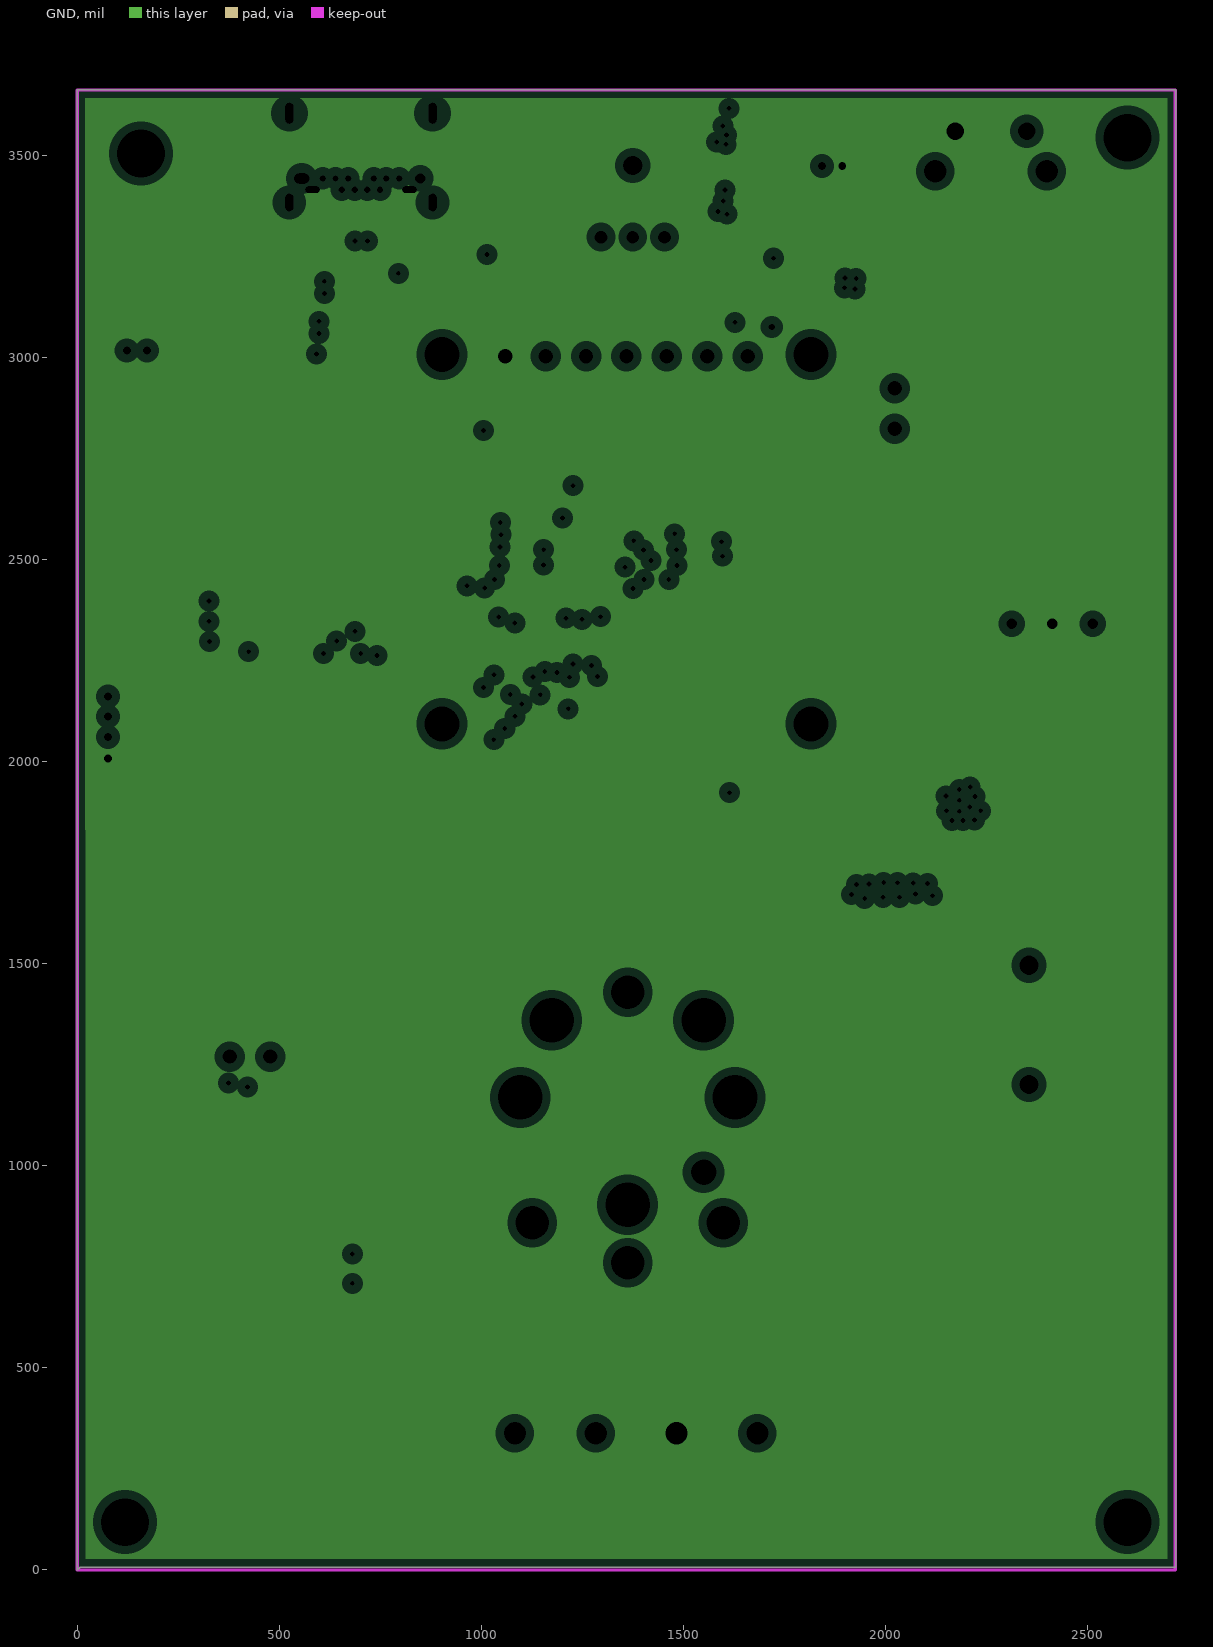
[diagram p0: GND, clearances drawn from the general rule]
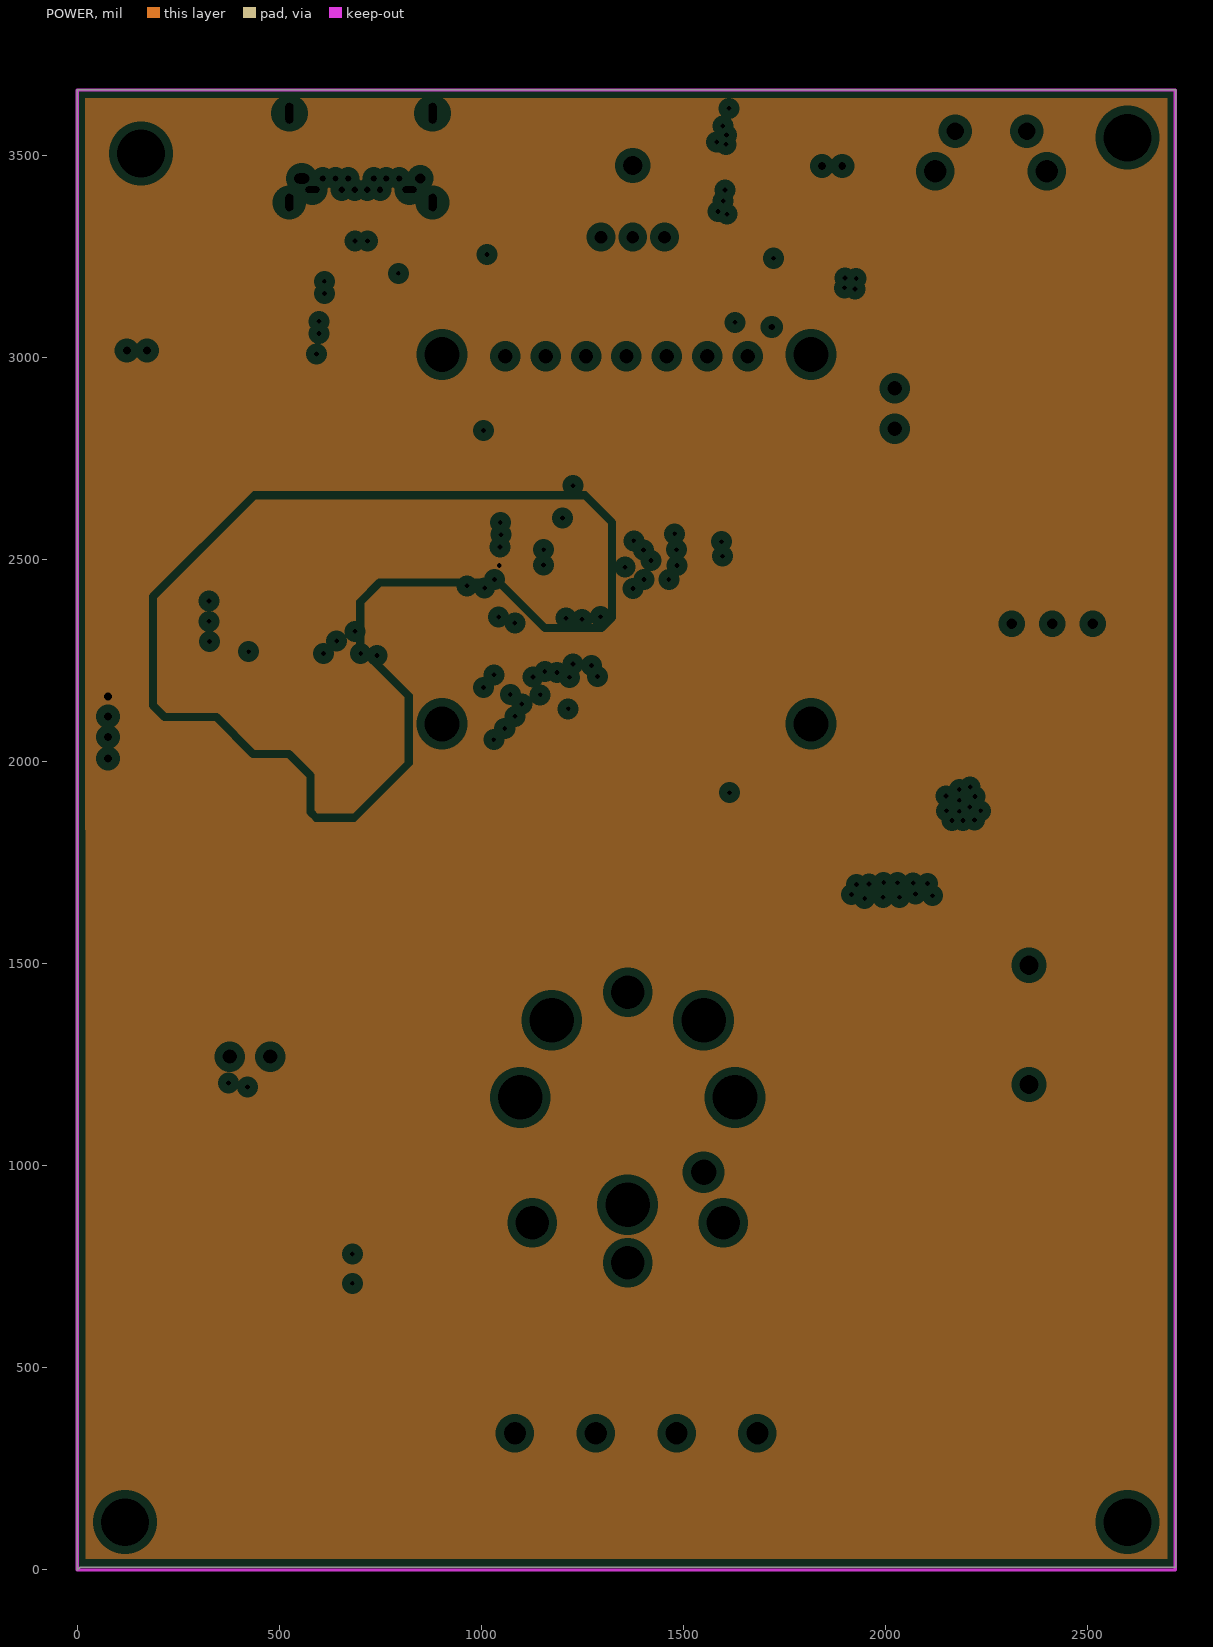
[diagram p1: POWER, clearances drawn from the general rule]
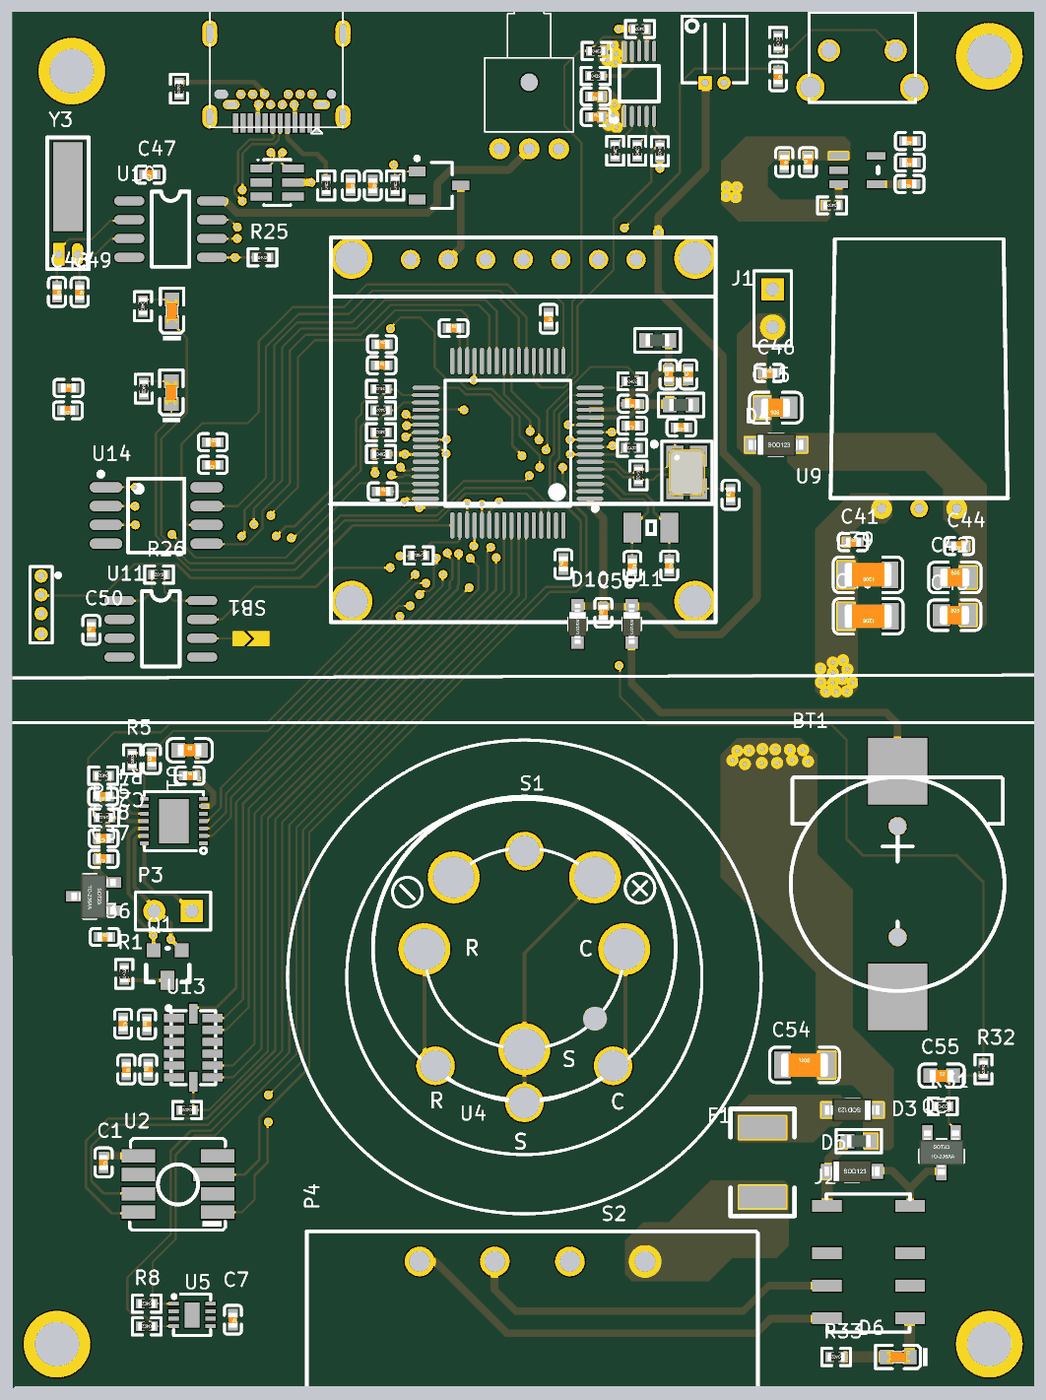
[diagram p2: 3D render of the assembled board from above, using the file's embedded part models]
# Altium PCB MISC105202.PcbDoc (part 2 of 3)
## Footprints (in the part's own frame and the unit in brackets; to place one, negate y for a bottom-side part, rotate by r counter-clockwise, add the part's x,y. Pads: shape width x height; smd on the part's side, far side on the other; paste and mask are expansions set on the pad) (continued)
SOT23-5 [mil]
  rect 20x50 smd: 1(74.8,100) 2(37.4,100) 3(0,100) 4(0,0) 5(74.8,0)
  silkscreen extent 30,-5 45,-5
SOT23-6 [mm] "SOT-23/SC-74A; 5 Leads; Body 3.1 x 3 mm, inc. leads (LxW max)"
  rect 0.55x1.45 smd: 1(-0.95,-1.075) 2(0,-1.075) 3(0.95,-1.075) 4(0.95,1.075) 5(0,1.075) 6(-0.95,1.075)
  silkscreen extent -1.57,-1.35 1.55,0.9
SOT-23 [mil]
  rect 36x36 smd: 1(0,0) 2(75,0)
  rect 36x50 smd: 3(38,80)
  silkscreen extent -20,-5 95,85
SOT-23(SOT-23-3) [mm]
  rect 1.25x0.7 smd: 1(1.25,-0.95) 2(1.25,0.95) 3(-1.25,0)
  silkscreen extent -0.65,-1.46 0.9,1.46, body extent -1.5,-1.5 1.5,1.5, height 1.3
SOT-23-3L [mm] "http://www.aosmd.com/res/packaging_information/SOT-23-3L.pdf"
  rect 1.15x0.65 smd: 1(1.475,-0.95) 2(1.475,0.95) 3(-1.475,0)
  silkscreen extent -0.9,-1.95 1.6,1.55, body extent -0.9,-1.55 0.9,1.55, height 1.25
USB_TYPEC [mm]
  oval 1x1.8 hole 0.5 slot 1.3 at 90 deg: 0(-4.5,-2.805) 0(4.5,-2.805)
  oval 1x1.6 hole 0.5 slot 1.1 at 90 deg: 0(-4.5,2.805) 0(4.5,2.805)
  round 0.61 hole 0.65 unplated: 0(-3.725,1.295)
  oval 0.64x0 hole 0.64 slot 0.95 at 0 deg unplated: 0(3.725,1.295)
  rect 0.35x1.3 smd: A1(-2.75,3.243) A2(-2.25,3.243) A3(-1.75,3.243) A4(-1.25,3.243) A5(-0.75,3.243) A6(-0.25,3.243) A7(0.25,3.243) A8(0.75,3.243) A9(1.25,3.243) A10(1.75,3.243) A11(2.25,3.243) A12(2.75,3.243)
  oval 1.14x0.64 hole 0.4 slot 0.9 at 0 deg: B1(3.05,1.995)
  round 0.65 hole 0.4: B2(2.4,1.295) B3(1.6,1.295) B4(1.2,1.995) B8(-0.8,1.295) B10(-1.6,1.295) B11(-2.4,1.295)
  round 0.64 hole 0.4: B5(0.8,1.295) B6(0.4,1.995) B7(-0.4,1.995) B9(-1.2,1.995)
  oval 1.15x0.65 hole 0.4 slot 0.9 at 0 deg: B12(-3.05,1.995)
  silkscreen extent -4.5,-6.46 4.5,3.96
WSON-14 [mm]
  rect 2x3 smd: 0(0,0)
  rect 0.6x0.254 smd: 1(-2,1.5) 2(-2,1) 3(-2,0.5) 4(-2,0) 5(-2,-0.5) 6(-2,-1) 7(-2,-1.5) 8(2,-1.5) 9(2,-1) 10(2,-0.5) 11(2,0) 12(2,0.5) 13(2,1) 14(2,1.5)
  silkscreen extent -2.2,-2 2,2.2
ZY78xxLS-1000 [mm]
  round 1.2 hole 0.65: 1(-2.54,0) 2(0,0) 3(2.54,0)
  silkscreen extent -6,0.69 6,18.2

## Part data
BT1: library part Battery, "Multicell Battery"
C1 C3 C4 C5 C7 C8 C10 C11 C12 C13 C14 C15 C16 C17 C18 C21 C22 C23 C24 C25 C26 C28 C31 C35 C47 C48 C49 C50 C51 C53: library part "Cap Semi", "Capacitor (Semiconductor SIM Model)"
C2: library part "0603 1uF (105) 10% 50V", "贴片电容"
C6 C9 C20 C27 C30 C52: library part "Cap Pol1", "Polarized Capacitor (Radial)"
C19: library part "0402 10nF (103) 10% 50V", "贴片电容"
C29 C33 C37 C41 C44 C46: library part "0402 100nF (104) 10% 16V", "贴片电容"
C32 C34 C36 C38: library part "0402 10uF (106) 20% 6.3V", "贴片电容"
C39 C40 C54: library part "1206 10uF (106) 10% 50V", "贴片电容"
C42 C43 C45: library part "0805 22uF (226) 20% 25V", "贴片电容"
C55: library part "0603 22uF (226) 20% 6.3V", "贴片电容"
C56: library part CAP, "Capacitor"
D1 D6: library part "0603 绿灯", "发光二极管"
D2: library part "0603 红灯", "发光二极管"
D3 D4 D5: library part "SOD-123 B5819W  SL", "肖特基二极管"
D10 D11: library part "SOD-323 1N4148WS T4", "二极管"
F1: library part "Fuse 2", "Fuse"
J1 P1 P3: library part "Header 2", "Header, 2-Pin"
L1 L2 L3: library part "0603 10uH 10%", "贴片电感"
OLED1: library part OLED_0.96
P2 P4: library part "Header 4", "Header, 4-Pin"
Q1: library part JFET
Q2: library part "AO3401A P道沟 X13A15 SOT-23", "MOS(场效应管)"
Q3: library part "SOT-23 SS8050 Y1", "三极管"
R1 R4: library part "0603 1.1KΩ (1101) 1%", "贴片电阻"
R2 R3 R5 R6 R8 R9 R10 R11 R12 R13 R14 R16 R17 R18 R19 R20 R21 R22 R23 R24 R25 R26 R27 R28 R29 R33: library part Reszte, "Resistor"
R7 R30: library part "0402 120Ω (1200) 1%", "贴片电阻"
R15: library part "0603 100Ω (1000) 1%", "贴片电阻"
R31: library part "0402 5.1KΩ (5101) 1%", "贴片电阻"
R32: library part "0402 680Ω (6800) 1%", "贴片电阻"
S2: library part 4NT
S3: library part SW-PB
SB1: library part JP2
U1: library part LMP91002
U3: library part TPS76901HDB
U6: "ARM"
U7: library part TPD4E001
U8: library part REF31xx
U9: library part ZY78xxLS
U11: library part SP706
U14: library part W25Q128FV
USB1: library part USB_Type_C_Receptacle
Y1: library part CRYSTAL_32K, "Crystal"
Y2: library part "SMD-3225_4P  16MHZ 9PF 10PPM", "贴片晶振"
Y3: library part XTAL_2P, "Crystal Oscillator"

## Free pads (board coordinates)
  round 177.17 hole 118.11: 0(118.11,118.11) 0(157.48,3503.94) 0(2598.43,118.11) 0(2598.43,3543.31)

## Via types
v1: diameter 24, hole 12, Top Layer to Bottom Layer, 107 vias
v2: diameter 30, hole 15, Top Layer to Bottom Layer, 1 vias

## Nets (pads, with @x,y where several pads share a name; then routed paths per layer and width w, separated by ;. In a path a pad name is that pad's centre, name@x,y a point inside that pad or via, vN(x,y) a via of type N, cw(c..) or ccw(c..) an arc to the next point about the centre after c; other vN are vias at no path point)
3V3: C1.1 C3.2 C4.2 C7.2 C9.1 C10.2 C11.2 C12.2 C13.2 C14.2 C17.2 C18.2 C20.1 C21.2 C27.1 C28.2 C30.1 C31.2 C33.2 C34.2 C47.2 C50.2 D10.1 L1.2 M1.2 M1.11 P2.1 Q2.2 R8.2 R9.2 R10.1 R11.2 R12.2 R16.2 R17.2 R19.1 R20.2 R21.2 R24.2 R25.2 R33.2 U1.6 U2.5 U3.5 U5.5 U6.19 U6.32 U6.64 U10.1 U11.2 U13.1 U13.6 U14.8 | length 272
  Top Layer w6: C1.1@245.67,617.72 C1.1@246.46,618.5
  Top Layer w12: C4.2@491,1628 C3.2@491,1687
  Top Layer w15: C4.2@487.73,1630 534,1583.73 534,1558 525,1549 U1.6@505,1549
  Top Layer w20: C1.1@246.46,618.5 U2.5@334.46,618.5
+5: C45.2 C46.1 C51.2 C52.1 D4.2 J1.2 U12.1 | length 898.7
  Top Layer w15: C51.2@1567.73,3382 C52.1@1567.73,3434.27 ; C51.2@1578.88,3384.12 U12.1@1625,3384.12
  Bottom Layer w20: v1@1599,3379 v1@1599,3384
  Bottom Layer w40: v1@1597,3379 1597,3279 1755,3121 1863,3121 1923,3061 1923,2922 J1.2@2022,2823
  other v1: 1607,3354 1585,3361 1598,3387 1602,3414
ADC1_IN1: C5.2 R5.2 U6.8 | length 1810.6
  Top Layer w6: R5.2@318.5,1690.35 C5.2@369.49,1690.35 ; C5.2@370.47,1690.75 428.54,1748.82 678.74,1748.82 997.31,2067.39 997.31,2067.61 1071.84,2142.13 v1(1099.61,2142.13) ; U6.8@1536.03,2504.34 1592.53,2504.34 v1(1596.06,2507.87)
  Bottom Layer w6: v1(1099.61,2142.13) v1@1101.57,2140.16 ; v1@1101.18,2139.76 1131.63,2109.31 1379.39,2109.31 1556.69,2286.61 1556.69,2468.5 v1(1596.06,2507.87)
ADC1_IN4: R15.2 U6.11 | length 2112.2
  Top Layer w6: R15.2@226.57,1518.9 226.57,1523.43 200.79,1549.21 200.79,1676.77 269.29,1745.28 394.88,1745.28 417.32,1767.72 673.62,1767.72 v1(1071.26,2165.35) ; v1(1477.94,2563.39) U6.11@1536.03,2563.39
  Bottom Layer w6: v1@1073.23,2165.35 v1(1071.26,2165.35) v1@1077.56,2165.35 ; v1@1077.56,2166.14 1112.6,2166.14 1142.52,2136.22 1187.4,2136.22 1194.49,2143.31 ; 1194.29,2143.5 1203.15,2152.36 1364.57,2152.36 1376.77,2164.57 ; 1376.97,2164.37 1526.38,2313.78 1526.38,2514.96 v1(1477.94,2563.39)
AGND: C5.1 C15.1 C29.1 C32.1 C36.1 C37.1 C38.1 L2.1 U1.0 U1.7 U6.12 U8.3 | length 336.2
  Top Layer w12: U6.12@1536.03,2583.08 1612.56,2583.08 1615.31,2585.82 1641.82,2585.82 C15.1@1666,2610 ; C15.1@1666,2614 C15.1@1666,2610 ; C15.1@1668,2612 C15.1@1666,2610
  Top Layer w25: C15.1@1668,2618 1737,2618 1748,2629 1748,2678.54 1746.27,2680.27 C29.1@1798,2680.27
ARM_TCK: P2.2 U6.49 | length 1191.6
  Top Layer w6: P2.2@86.22,2109.06 239.97,2109.06 323.83,2192.91 437.01,2192.91 474.02,2155.91 765.35,2155.91 905.13,2295.68 U6.49@1169.89,2295.68
ARM_TMS: P2.3 U6.46 | length 1218.4
  Top Layer w6: v1(424.02,2271.65) 485.43,2210.24 725.98,2210.24 923.76,2408.02 977.16,2408.02 1096.92,2408.02 U6.46@1099.02,2405.91
  Bottom Layer w6: P2.3@75.98,2061.42 136.22,2061.42 258.66,2183.86 336.22,2183.86 v1(424.02,2271.65)
AVCC: C15.2 C29.2 C32.2 C36.2 L1.1 R1.2 U6.13 U8.1 | length 375.5
  Top Layer w10: C15.2@1633,2618 C15.2@1634,2619
  Top Layer w12: U6.13@1536.03,2602.76 1537.09,2603.82 1600.82,2603.82 1615,2618 C15.2@1631,2618 ; C15.2@1633,2616 C15.2@1634,2617
  Top Layer w20: C15.2@1632.87,2619.68 1638.53,2625.34 1638.53,2639.11 1649.36,2649.94 1686.94,2649.94 1708,2671 1708,2693 1728,2713 ; L1.1@1745,2780 1745,2717 1749,2713 C29.2@1797,2713
BAT_CHG: R27.1 U6.20 U12.8 | length 1225.7
  Top Layer w6: U6.20@1406.11,2732.69 1406.11,2689.56 1416.14,2679.53 1465.75,2679.53 1488.98,2702.76 1488.98,2891.73 1512.99,2915.75 1512.99,3314.57 1467.72,3359.84 1467.72,3507.87 ; 1468.5,3507.87 1468.11,3507.87 1468.11,3516.92 1508.27,3557.09 R27.1@1534.25,3557.09 ; R27.1@1537.2,3557.48 1537.2,3561.35 R27.1@1541.73,3565.88 ; R27.1@1541.73,3565.75 R27.1@1541.73,3565.88 ; U12.8@1667.32,3575.98 1667.32,3584.25 1657.64,3593.94 1569.79,3593.94 R27.1@1541.73,3565.88
BAT_PG: R2.1 U6.21 U12.5 | length 940.1
  Top Layer w6: U6.21@1386.43,2732.69 1386.43,2681.68 1405.51,2662.6 1466.49,2662.6 1502.76,2698.86 1502.76,2879.53 1598.82,2975.59 1598.82,3110.24 1699.43,3210.85 1699.43,3230 1699.43,3249 1700.2,3249.77 1700.2,3289.81 1711.4,3301 R2.1@1716,3301 ; U12.5@1706.3,3360.63 1706.3,3349.21 1721,3334.51 R2.1@1721,3310
D_N: U6.44 U7.6 USB1.A7 USB1.B7 | length 1866.1
  Top Layer w6: v1(611.3,3158) 590,3179.3 590,3196.7 600,3206.7 600,3290.97 631.03,3322 691,3322 695.78,3326.78 695.78,3332.92 691.94,3336.76 USB1.A7@691.94,3365.69 ; 709.45,3264.96 729.13,3245.28 U7.6@746.26,3245.28 ; 709.98,3265.49 v1@709.98,3284.78 ; 1040.84,2441.44 1056.66,2441.44 1060.5,2445.28 U6.44@1099.02,2445.28
  Bottom Layer w6: v1@611,3157 602,3166 564,3166 532,3134 532,2994 579,2947 679.42,2947 792.77,2833.65 905.76,2833.65 938.98,2800.43 938.98,2529.41 1017.99,2450.39 v1(1031.89,2450.39) ; v1@613.15,3156.15 623.14,3166.14 676.42,3166.14 708.85,3198.57 708.85,3274.99 v1@716.93,3283.07 ; v1@708.01,3290.81 708.01,3316.11 708,3402.88 USB1.B7@716.54,3411.42
  other v1: 717.72,3287.4
D_P: U6.45 U7.1 USB1.A6 USB1.B6 | length 1838.5
  Top Layer w6: v1@612,3189 612,3286 636,3310 695.97,3310 707.78,3321.81 707.78,3332.92 711.62,3336.76 USB1.A6@711.62,3365.69 ; U7.1@661.61,3245.28 676.38,3245.28 695.28,3264.17 v1@695.28,3281.5 ; v1@1012.99,2424.41 1037.49,2424.41 1042.52,2429.44 1056.66,2429.44 1060.5,2425.6 U6.45@1099.02,2425.6
  Bottom Layer w6: v1@608.87,3188 598.87,3178 559.03,3178 520,3138.97 520,2989.03 574.03,2935 674.45,2935 787.8,2821.65 900.79,2821.65 926.98,2795.46 926.98,2524.44 1007.87,2443.54 v1(1007.87,2429.53) ; v1@615,3185 621.86,3178.14 671.45,3178.14 696.85,3203.54 696.85,3271.65 v1@691.73,3276.77 ; USB1.B6@687.8,3412.2 695.67,3404.33 v1@695.67,3294.88
  other v1: 611,3188 687.01,3287.4
DRDY: U6.55
Gas_3_CE: P3.1 S1.1 S2.1 U1.14 U4.2 | length 1807.5
  Top Layer w10: U1.14@350.39,1450.39 350.39,1347.61 382,1316 428,1316 P3.1@462,1282 ; S2.1@1597.64,858.58 1630,890.95 1630,1174 S1.1@1624,1180
  Bottom Layer w10: P3.1@477,1270 809,1270 815,1270 1090,1270 U4.2@1162,1342 ; U4.2@1190,1362 1390,1162 S1.1@1621,1162
Gas_3_RE: P3.2 Q1.1 S1.3 S2.3 U1.13 | length 1327.5
  Top Layer w10: U1.13@347,1470 332,1470 324,1462 324,1334 421,1237 v1(421,1195) Q1.1@450,1166 ; S1.3@1095.67,1168.8 1095.67,895.33 S2.3@1125,866
  Bottom Layer w10: v1(421,1195) S1.3@1059,1195
Gas_3_WE: Q1.2 S1.2 S2.2 U1.12 U4.1 | length 2107.8
  Top Layer w10: U1.12@350.39,1489.76 326.76,1489.76 308,1471 308,1317 329,1296 329,1252 v1@375,1206 ; v1(374,1205) v1@375,1206 ; Q1.2@375,1166 v1@375,1206 ; S2.2@1361.42,760.16 S1.2@1361.42,903.06 1361.42,1158.42 U4.1@1541,1338
  Bottom Layer w10: v1(374,1205) 424,1155 940,1155 1053,1042 1225,1042 S1.2@1333,934
Gas_MENB: U1.2 U6.9 | length 1665.3
  Top Layer w6: U1.2@507.87,1470.08 532.28,1470.08 581,1518.8 581,1572.34 1143.7,2135.04 v1@1143.7,2162.6 ; v1(1482.67,2524.02) U6.9@1536.03,2524.02
  Bottom Layer w6: v1@1145.28,2168.11 1146.85,2169.68 1357.87,2169.68 1509.84,2321.65 1509.84,2496.85 v1(1482.67,2524.02)
  other v1: 1145.28,2164.96
Gas_SCL: R20.1 U1.3 U6.34 | length 1861
  Top Layer w6: U1.3@507.87,1489.76 524.41,1489.76 568,1533.35 568,1582.17 v1@1030.31,2044.49 ; v1(701.18,2267.32) 727.17,2293.31 750.79,2293.31 913.78,2456.3 913.78,2577.95 927.95,2592.13 927.95,2619.29 940.16,2631.5 973.36,2631.5 996.65,2654.79 R20.1@996.65,2658.66 ; R20.1@1001.57,2657.48 1020.87,2657.48 1036.21,2642.13 U6.34@1099.02,2642.13
  Bottom Layer w6: v1(701.18,2267.32) 793.7,2174.8 929.92,2174.8 1029.92,2074.8 v1@1029.92,2053.94
  other v1: 1030.31,2053.94
Gas_SDA: R21.1 U1.4 U6.35 | length 1782.1
  Top Layer w6: U1.4@507.87,1509.45 519.29,1509.45 554,1544.16 554,1596.91 1009.31,2052.23 1009.31,2062.64 1028.18,2081.5 1057.09,2081.5 v1(1057.48,2081.89) ; v1(741.34,2262.2) 747.24,2262.2 925.98,2440.94 925.98,2557.48 945.28,2576.77 975.72,2576.77 997.05,2598.1 R21.1@997.05,2601.57 ; R21.1@996.46,2601.57 R21.1@997.05,2601.57 ; R21.1@997.05,2601.97 R21.1@997.05,2601.57 ; U6.35@1099.02,2622.45 1039.38,2622.45 1018.5,2601.57 R21.1@997.05,2601.57
  Bottom Layer w6: v1(741.34,2262.2) 808.27,2195.28 933.46,2195.28 v1@1046.85,2081.89
GND: BT1.2 C1.2 C3.1 C4.1 C6.2 C7.1 C8.2 C9.2 C10.1 C11.1 C12.1 C13.1 C14.1 C16.1 C17.1 C18.1 C19.2 C20.2 C21.1 C22.1 C23.1 C24.1 C25.1 C26.1 C27.2 C28.1 C30.2 C31.1 C33.1 C34.1 C35.1 C39.1 C40.1 C41.2 C42.1 C43.1 C44.2 C45.1 C46.2 C47.1 C48.2 C49.2 C50.1 C51.1 C52.2 C53.2 C54.1 C55.1 C56.1 J2.6 L2.2 M1.5 M1.8 OLED1.1 P1.2 P2.4 P4.2 Q3.2 R3.1 R22.2 R23.1 R28.1 R29.1 R31.1 S3.2 U1.1 U2.2 U2.6 U3.2 U5.0 U5.2 U5.7 U5.8 U6.18 U6.60 U6.63 U7.2 U9.2 U10.4 U11.3 U12.3 U13.2 U13.4 U13.5 U13.11 U14.4 USB1.A1 USB1.A12 USB1.B1 USB1.B12
GND-P: 
I2C1_SCL: R9.1 U5.4 U6.58 | length 2681.4
  Top Layer w6: U5.4@420.08,166.14 378.74,166.14 352.76,192.13 324.41,192.13 305.12,211.42 305.12,294.88 420.08,409.84 420.08,631.5 474.02,685.43 528.35,685.43 736,893.09 736,1498.6 1347.06,2109.65 U6.58@1347.06,2295.68
I2C1_SDA: R8.1 U5.1 U6.59 | length 2557.2
  Top Layer w6: R8.1@372.83,231.89 372.83,337.4 433.86,398.43 433.86,622.05 484.25,672.44 537.4,672.44 755,890.04 755,1491.22 1365.84,2102.06 1365.84,2294.78 U6.59@1366.74,2295.68 ; R8.1@377.95,225.2 378.35,225.59 U5.1@428.35,225.59
INT1: U6.24 U13.8 | length 2359.3
  Top Layer w6: U13.8@531.89,827.95 587.01,827.95 662,902.94 662,1522.24 1262.99,2123.23 1262.99,2225.98 v1@1272.05,2235.04 ; U6.24@1327.37,2732.69 1327.37,2652.16 1400.39,2579.13 v1(1400.39,2523.62) ; v1@1400.39,2523.23 v1(1400.39,2523.62) ; v1@1401.18,2523.62 v1(1400.39,2523.62)
  Bottom Layer w6: v1(1272.05,2237.8) 1291.34,2237.8 1334.12,2280.57 1334.12,2495.93 1350.39,2512.2 1388.98,2512.2 v1(1400.39,2523.62)